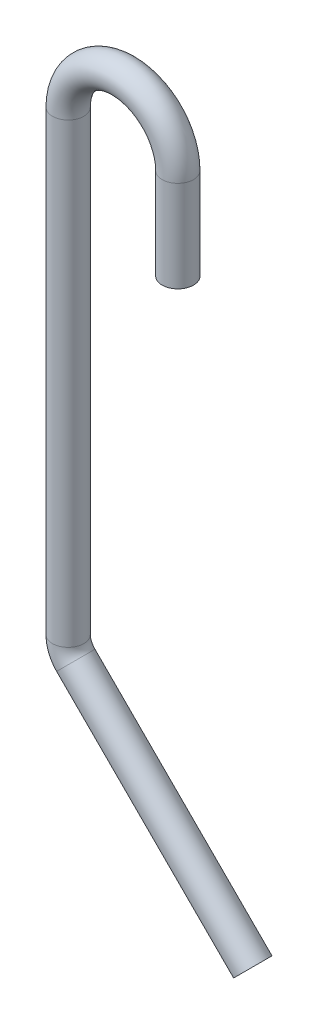
from build123d import *

# Parameters (mm, degrees)
SWEEP_1_PROFILE_R = 6


with BuildPart() as part:
    # 扫描1: sweep along a path in 草图1
    with BuildLine(Plane.XY) as sweep_1_path:
        Line((0, 0), (-67.781745931, 67.781745931))
        ThreePointArc((-67.781745931, 67.781745931), (-69.949473444, 71.025979419), (-70.710678119, 74.852813742))
        Line((-70.710678119, 74.852813742), (-70.710678119, 249.710678119))
        ThreePointArc((-70.710678119, 249.710678119), (-49.710678119, 270.710678119), (-28.710678119, 249.710678119))
        Line((-28.710678119, 249.710678119), (-28.710678119, 214.710678119))
    # 扫描1 profile (on start of the path) → 扫描1 (sweep)
    with BuildSketch(Plane(origin=(0, 0, 0), x_dir=(-0.7071067811865462, -0.7071067811865488, 0), z_dir=(-0.7071067811865488, 0.7071067811865462, 0))):
        Circle(SWEEP_1_PROFILE_R)
    sweep(path=sweep_1_path.line)


solid = part.part
